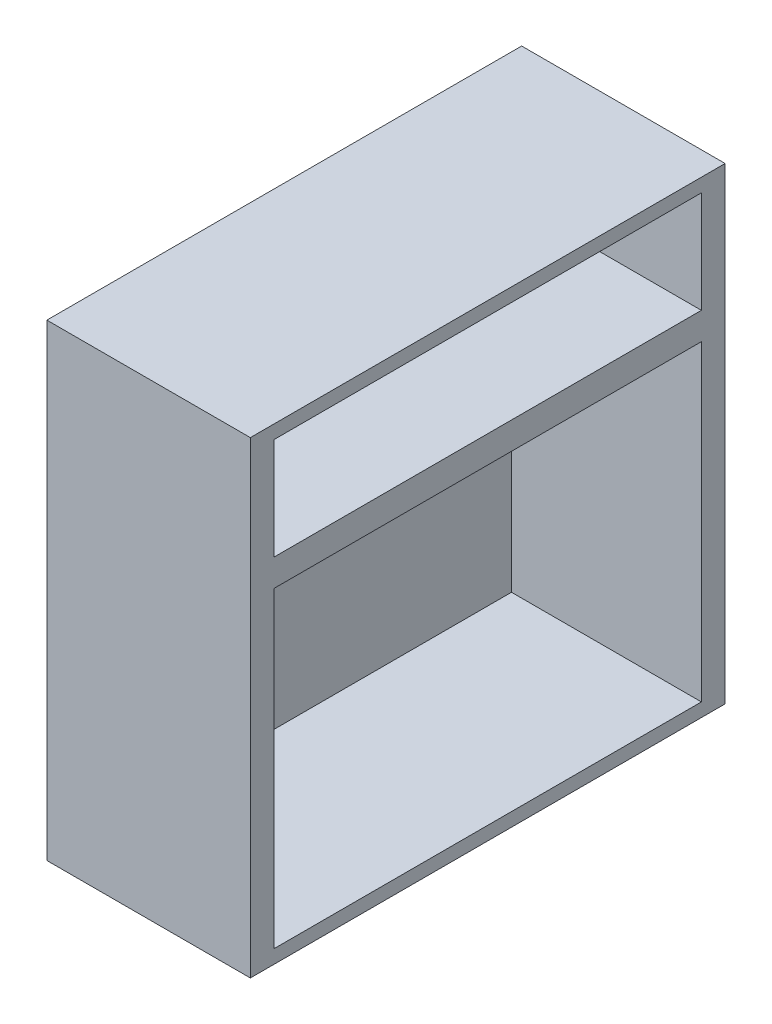
SolidWorks part; units mm, degrees
material "Q235A"
ref_plane "Front Plane" through (0, 0, 0) normal (0, 0, 1) x (1, 0, 0)
ref_plane "Top Plane" through (0, 0, 0) normal (0, 1, 0) x (1, 0, 0)
ref_plane "Right Plane" through (0, 0, 0) normal (1, 0, 0) x (0, 0, -1)
sketch "Sketch1" plane through (0, 0, 0) normal (0, 0, 1) x (1, 0, 0)
  line L1 (150, -345) -> (-150, -345)
  line L2 (150, -345) -> (150, 345)
  line L3 (150, 345) -> (-150, 345)
  line L4 (-150, -345) -> (-150, 345)
  line L5 (150, -345) -> (-150, 345) construction
  line L6 (150, 345) -> (-150, -345) construction
  point P0 (0, 0)
  dimension "D1" = 300
  dimension "D2" = 690
extrude "Boss-Extrude1" add sketch "Sketch1" along normal blind 700
sketch "Sketch2" plane through (150, 0, 0) normal (1, 0, 0) x (0, 0, -1)
  line L0 (-700, 345) -> (0, 345) construction
  line L1 (-35, 175) -> (-665, 175)
  line L2 (-35, 175) -> (-35, 325)
  line L3 (-35, 325) -> (-665, 325)
  line L4 (-665, 175) -> (-665, 325)
  line L5 (-35, 175) -> (-665, 325) construction
  line L6 (-35, 325) -> (-665, 175) construction
  line L7 (0, -345) -> (0, 345) construction
  line L8 (-700, -345) -> (-700, 345) construction
  point P0 (-350, 250)
  dimension "D1" = 20
  dimension "D2" = 35
  dimension "D3" = 35
  dimension "D4" = 150
extrude "Cut-Extrude1" cut sketch "Sketch2" against normal blind 280
sketch "Sketch3" plane through (150, 0, 0) normal (1, 0, 0) x (0, 0, -1)
  line L0 (-665, 325) -> (-665, 175) construction
  line L1 (-35, -325) -> (-665, -325)
  line L2 (-35, -325) -> (-35, 135)
  line L3 (-35, 135) -> (-665, 135)
  line L4 (-665, -325) -> (-665, 135)
  line L5 (-35, -325) -> (-665, 135) construction
  line L6 (-35, 135) -> (-665, -325) construction
  line L7 (-35, 175) -> (-35, 325) construction
  line L8 (-700, -345) -> (0, -345) construction
  line L9 (-665, 175) -> (-35, 175) construction
  point P0 (-350, -95)
  dimension "D1" = 20
  dimension "D2" = 40
extrude "Cut-Extrude2" cut sketch "Sketch3" against normal blind 280
